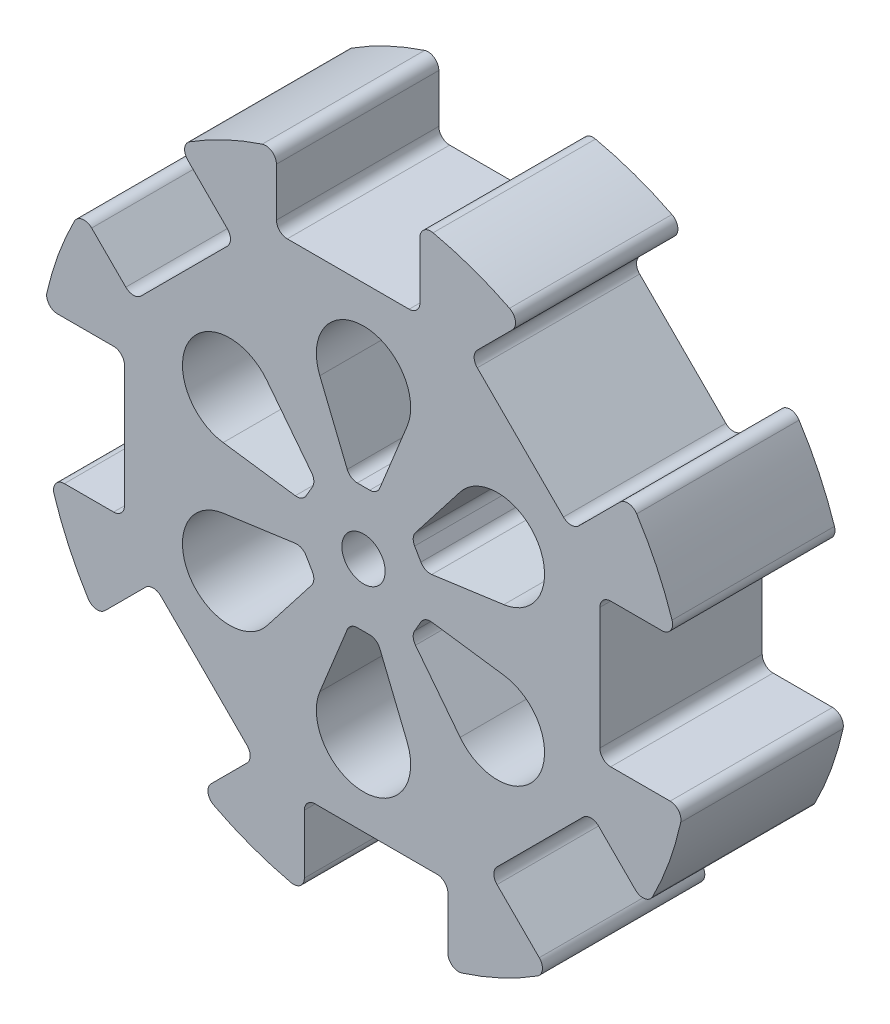
from build123d import *

# Parameters (mm, degrees)
SKETCH1_R                = 4
BOSS_EXTRUDE2_DEPTH      = 30
CUT_EXTRUDE2_DEPTH       = 89.20573662
FILLET1_R                = 2
CIRPATTERN1_COUNT        = 6
FILLET1_OF_CIRPATTERN1_R = 2
SKETCH12_R               = 0.68344787
CUT_EXTRUDE4_DEPTH       = 1


with BuildPart() as part:
    # Sketch1 → Boss-Extrude2 (new body)
    with BuildSketch(Plane.XY):
        with BuildLine():
            Line((10.429173845, 56.65258721), (10.429173845, 46.168579918))
            ThreePointArc((10.429173845, 46.168579918), (9.843387407, 44.754366355), (8.429173845, 44.168579918))
            Line((8.429173845, 44.168579918), (-14.085800573, 44.168579918))
            ThreePointArc((-14.085800573, 44.168579918), (-15.500014135, 44.754366355), (-16.085800573, 46.168579918))
            Line((-16.085800573, 46.168579918), (-16.085800573, 55.108110271))
            ThreePointArc((-16.085800573, 55.108110271), (-16.912620406, 56.727878247), (-18.709448869, 57.008389935))
            ThreePointArc((-18.709448869, 57.008389935), (-25.61401293, 54.257924229), (-32.125557949, 50.67492996))
            ThreePointArc((-32.125557949, 50.67492996), (-33.042575786, 49.205706038), (-32.46891958, 47.571552066))
            Line((-32.46891958, 47.571552066), (-25.168022999, 40.270655485))
            ThreePointArc((-25.168022999, 40.270655485), (-24.582236562, 38.856441923), (-25.168022999, 37.44222836))
            Line((-25.168022999, 37.44222836), (-41.088514088, 21.521737271))
            ThreePointArc((-41.088514088, 21.521737271), (-42.50272765, 20.935950834), (-43.916941213, 21.521737271))
            Line((-43.916941213, 21.521737271), (-50.22249286, 27.827288919))
            ThreePointArc((-50.22249286, 27.827288919), (-51.948014566, 28.38869861), (-53.417282506, 27.323871059))
            ThreePointArc((-53.417282506, 27.323871059), (-56.386758875, 20.506911606), (-58.490248558, 13.375007425))
            ThreePointArc((-58.490248558, 13.375007425), (-58.10448971, 11.682511734), (-56.540573606, 10.929173845))
            Line((-56.540573606, 10.929173845), (-46.168579918, 10.929173845))
            ThreePointArc((-46.168579918, 10.929173845), (-44.754366355, 10.343387407), (-44.168579918, 8.929173845))
            Line((-44.168579918, 8.929173845), (-44.168579918, -13.585800573))
            ThreePointArc((-44.168579918, -13.585800573), (-44.754366355, -15.000014135), (-46.168579918, -15.585800573))
            Line((-46.168579918, -15.585800573), (-55.269698915, -15.585800573))
            ThreePointArc((-55.269698915, -15.585800573), (-56.884135943, -16.405295137), (-57.175550602, -18.192207489))
            ThreePointArc((-57.175550602, -18.192207489), (-54.452420305, -25.197895208), (-50.874763654, -31.808150263))
            ThreePointArc((-50.874763654, -31.808150263), (-49.405090867, -32.735051195), (-47.764724636, -32.16209215))
            Line((-47.764724636, -32.16209215), (-40.270655485, -24.668022999))
            ThreePointArc((-40.270655485, -24.668022999), (-38.856441923, -24.082236562), (-37.44222836, -24.668022999))
            Line((-37.44222836, -24.668022999), (-21.521737271, -40.588514088))
            ThreePointArc((-21.521737271, -40.588514088), (-20.935950834, -42.00272765), (-21.521737271, -43.416941213))
            Line((-21.521737271, -43.416941213), (-28.157199739, -50.05240368))
            ThreePointArc((-28.157199739, -50.05240368), (-28.719595437, -51.771602209), (-27.665158113, -53.241328182))
            ThreePointArc((-27.665158113, -53.241328182), (-20.687232491, -56.320852372), (-13.375007425, -58.490248558))
            ThreePointArc((-13.375007425, -58.490248558), (-11.682511734, -58.10448971), (-10.929173845, -56.540573606))
            Line((-10.929173845, -56.540573606), (-10.929173845, -45.668579918))
            ThreePointArc((-10.929173845, -45.668579918), (-10.343387407, -44.254366355), (-8.929173845, -43.668579918))
            Line((-8.929173845, -43.668579918), (13.585800573, -43.668579918))
            ThreePointArc((13.585800573, -43.668579918), (15.000014135, -44.254366355), (15.585800573, -45.668579918))
            Line((15.585800573, -45.668579918), (15.585800573, -55.269698915))
            ThreePointArc((15.585800573, -55.269698915), (16.405295137, -56.884135943), (18.192207489, -57.175550602))
            ThreePointArc((18.192207489, -57.175550602), (25.3679699, -54.373395178), (32.125557949, -50.67492996))
            ThreePointArc((32.125557949, -50.67492996), (33.042575786, -49.205706038), (32.46891958, -47.571552066))
            Line((32.46891958, -47.571552066), (24.668022999, -39.770655485))
            ThreePointArc((24.668022999, -39.770655485), (24.082236562, -38.356441923), (24.668022999, -36.94222836))
            Line((24.668022999, -36.94222836), (40.588514088, -21.021737271))
            ThreePointArc((40.588514088, -21.021737271), (42.00272765, -20.435950834), (43.416941213, -21.021737271))
            Line((43.416941213, -21.021737271), (50.22249286, -27.827288919))
            ThreePointArc((50.22249286, -27.827288919), (51.948014566, -28.38869861), (53.417282506, -27.323871059))
            ThreePointArc((53.417282506, -27.323871059), (56.476791597, -20.257640804), (58.6061247, -12.857766046))
            ThreePointArc((58.6061247, -12.857766046), (58.210981319, -11.175615789), (56.65258721, -10.429173845))
            Line((56.65258721, -10.429173845), (45.668579918, -10.429173845))
            ThreePointArc((45.668579918, -10.429173845), (44.254366355, -9.843387407), (43.668579918, -8.429173845))
            Line((43.668579918, -8.429173845), (43.668579918, 14.085800573))
            ThreePointArc((43.668579918, 14.085800573), (44.254366355, 15.500014135), (45.668579918, 16.085800573))
            Line((45.668579918, 16.085800573), (55.108110271, 16.085800573))
            ThreePointArc((55.108110271, 16.085800573), (56.727878247, 16.912620406), (57.008389935, 18.709448869))
            ThreePointArc((57.008389935, 18.709448869), (54.177712128, 25.783240847), (50.473399603, 32.441268972))
            ThreePointArc((50.473399603, 32.441268972), (49.004687645, 33.348439914), (47.376739387, 32.774106902))
            Line((47.376739387, 32.774106902), (39.770655485, 25.168022999))
            ThreePointArc((39.770655485, 25.168022999), (38.356441923, 24.582236562), (36.94222836, 25.168022999))
            Line((36.94222836, 25.168022999), (21.021737271, 41.088514088))
            ThreePointArc((21.021737271, 41.088514088), (20.435950834, 42.50272765), (21.021737271, 43.916941213))
            Line((21.021737271, 43.916941213), (27.495609263, 50.390813204))
            ThreePointArc((27.495609263, 50.390813204), (28.056010613, 52.122667993), (26.980754173, 53.591407))
            ThreePointArc((26.980754173, 53.591407), (20.076448185, 56.541455838), (12.857766046, 58.6061247))
            ThreePointArc((12.857766046, 58.6061247), (11.175615789, 58.210981319), (10.429173845, 56.65258721))
        make_face()
        Circle(SKETCH1_R, mode=Mode.SUBTRACT)
    extrude(amount=BOSS_EXTRUDE2_DEPTH)

    # Sketch2 → Cut-Extrude2 (cut, symmetric)
    with BuildSketch(Plane.XY.offset(30)):
        with BuildLine():
            Line((-2.5, 11.575217828), (2.5, 11.575217828))
            Line((2.5, 11.575217828), (8.072844982, 25.27762882))
            ThreePointArc((8.072844982, 25.27762882), (0, 37.27586788), (-8.072844982, 25.27762882))
            Line((-8.072844982, 25.27762882), (-2.5, 11.575217828))
        make_face()
    cut_extrude2 = extrude(amount=CUT_EXTRUDE2_DEPTH, both=True, mode=Mode.SUBTRACT)

    # Fillet1
    fillet1_edges = [part.edges().sort_by_distance(p)[0] for p in [
        (-2.5, 11.575217828, 15),
        (2.5, 11.575217828, 15),
    ]]
    fillet(fillet1_edges, radius=FILLET1_R)

    # CirPattern1: Cut-Extrude2 ×6 about axis
    cirpattern1_axis = Axis((0, 0, 0), (0, 0, 1))
    for i in range(1, CIRPATTERN1_COUNT):
        add(cut_extrude2.rotate(cirpattern1_axis, i * 360 / CIRPATTERN1_COUNT), mode=Mode.SUBTRACT)

    # Fillet1 of CirPattern1
    fillet1_of_cirpattern1_edges = [part.edges().sort_by_distance(p)[0] for p in [
        (-11.274432693, 3.622545404, 15),
        (-8.774432693, 7.952672423, 15),
        (-8.774432693, -7.952672423, 15),
        (-11.274432693, -3.622545404, 15),
        (2.5, -11.575217828, 15),
        (-2.5, -11.575217828, 15),
        (11.274432693, -3.622545404, 15),
        (8.774432693, -7.952672423, 15),
        (8.774432693, 7.952672423, 15),
        (11.274432693, 3.622545404, 15),
    ]]
    fillet(fillet1_of_cirpattern1_edges, radius=FILLET1_OF_CIRPATTERN1_R)

    # Sketch12 → Cut-Extrude4 (cut)
    with BuildSketch(Plane(origin=(0, 0, 0), x_dir=(-1, 0, 0), z_dir=(0, 0, -1))):
        with Locations((32.110275417, -0.556072549)):
            Circle(SKETCH12_R)
    extrude(amount=-CUT_EXTRUDE4_DEPTH, mode=Mode.SUBTRACT)


solid = part.part
